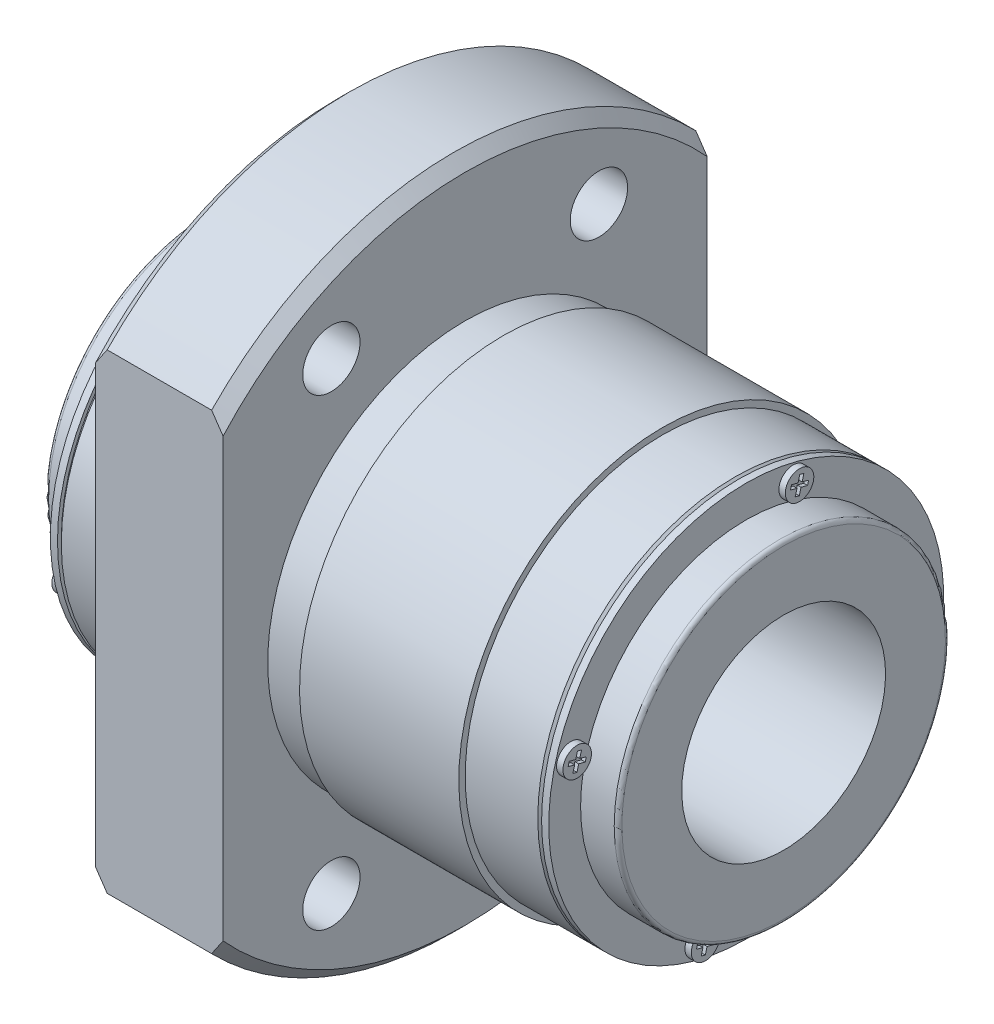
SolidWorks part; units mm, degrees
ref_plane "Front" through (0, 0, 0) normal (0, 0, 1) x (1, 0, 0)
ref_plane "Top" through (0, 0, 0) normal (0, 1, 0) x (1, 0, 0)
ref_plane "Right" through (0, 0, 0) normal (1, 0, 0) x (0, 0, -1)
sketch "Sketch1" plane through (0, 0, 0) normal (0, 0, 1) x (1, 0, 0)
  line L0 (35, 8) -> (-10, 8)
  line L1 (-10, 8) -> (-10, 13)
  line L2 (-10, 13) -> (-7.06, 13)
  line L3 (-7.06, 13) -> (-7.06, 15.5)
  line L4 (-7.06, 15.5) -> (-0.65, 15.5)
  line L5 (-0.65, 15.5) -> (-0.65, 16)
  line L6 (-0.65, 16) -> (0, 16)
  line L7 (0, 16) -> (0, 26.5)
  line L8 (0, 26.5) -> (10, 26.5)
  line L9 (10, 26.5) -> (10, 15.5)
  line L10 (10, 15.5) -> (13, 15.5)
  line L11 (13, 15.5) -> (13, 16)
  line L12 (13, 16) -> (25.5, 16)
  line L13 (25.5, 16) -> (25.5, 15.5)
  line L14 (25.5, 15.5) -> (32.06, 15.5)
  line L15 (32.06, 15.5) -> (32.06, 13)
  line L16 (32.06, 13) -> (35, 13)
  line L17 (35, 13) -> (35, 8)
  line L18 (35, 0) -> (-10, 0) construction
  dimension "D1" = 0.65
  dimension "D2" = 7.06
  dimension "D3" = 10
  dimension "D4" = 10
  dimension "D5" = 13
  dimension "D6" = 25.5
  dimension "D7" = 32.06
  dimension "D8" = 35
  dimension "D9" = 16
  dimension "D10" = 26
  dimension "D11" = 31
  dimension "D12" = 32
  dimension "D13" = 53
revolve "Revolve1" add sketch "Sketch1" angle 360 about L18
sketch "Sketch2" plane through (0, 0, 0) normal (1, 0, 0) x (0, 0, -1)
  line L0 (0, 26.5) -> (0, -26.5) construction
  line L1 (-19, 26.5) -> (19, 26.5)
  line L2 (-19, 26.5) -> (-19, -26.5)
  line L3 (-19, -26.5) -> (19, -26.5)
  line L4 (19, 26.5) -> (19, -26.5)
  circle A0 centre (0, 0) radius 26.5 construction
  dimension "D1" = 38
extrude "Cut-Extrude1" cut sketch "Sketch2" along normal through all flip side to cut
hole_wizard "Ø4.5 (4.5) Diameter Hole1" positions "Sketch5" profile "Sketch4" hole size "Ø4.5" standard "ISO" end condition through all
sketch "Sketch5" plane through (10, 0, 0) normal (1, 0, 0) x (0, 0, -1)
  line L1 (0, 26.5) -> (0, -21) construction
  circle A0 centre (0, 0) radius 21 construction
  arc A3 (19, 18.473) -> (-19, 18.473) centre (0, 0) ccw construction
  point P0 (-10.5, 18.1865)
  point P1 (-10.5, -18.1865)
  point P3 (10.5, 18.1865)
  point P5 (10.5, -18.1865)
  dimension "D1" = 42
  dimension "D2" = 21
sketch "Sketch4" plane through (10, 18.1865, 10.5) normal (0, 1, 0) x (0, 0, -1)
  line L0 (0, 0) -> (0, 20)
  line L1 (0, 20) -> (2.25, 20)
  line L2 (2.25, 20) -> (2.25, 0)
  line L5 (2.25, 0) -> (0, 0)
  line L11 (0, -6.35) -> (0, 107.95) construction
  dimension "Thru Hole Dia." = 4.5
  dimension "Thru Hole Depth" = 20
sketch "Sketch6" plane through (32.06, 0, 0) normal (1, 0, 0) x (0, 0, -1)
  line L0 (-19, 0) -> (19, 0) construction
  line L1 (0, 26.5) -> (0, -26.5) construction
  line L2 (-18.1829, 4.8721) -> (18.5076, -4.9591) construction
  line L3 (-4.9176, -18.3528) -> (4.686, 17.4885) construction
  line L4 (-19, -18.473) -> (-19, 18.473) construction
  line L5 (19, 18.473) -> (19, -18.473) construction
  circle A0 centre (0, 0) radius 14.25 construction
  circle A3 centre (3.6882, 13.7644) radius 1.12
  circle A4 centre (-13.7644, 3.6882) radius 1.12
  circle A5 centre (-3.6882, -13.7644) radius 1.12
  circle A6 centre (13.7644, -3.6882) radius 1.12
  arc A7 (19, 18.473) -> (-19, 18.473) centre (0, 0) ccw construction
  arc A8 (-19, -18.473) -> (19, -18.473) centre (0, 0) ccw construction
  dimension "D1" = 28.5
  dimension "D2" = 2.24
  dimension "D3" = 15
  dimension "D4" = 75
extrude "Boss-Extrude1" add sketch "Sketch6" along normal blind 0.5
sketch "Sketch7" plane through (32.56, 0, 0) normal (1, 0, 0) x (0, 0, -1)
  line L0 (-4.9176, -18.3528) -> (4.686, 17.4885) construction
  line L1 (4.0274, 14.3931) -> (3.7087, 14.4785)
  line L2 (4.0274, 14.3931) -> (3.8903, 13.8811)
  line L3 (3.6677, 13.0504) -> (3.3489, 13.1358)
  line L4 (3.7087, 14.4785) -> (3.5715, 13.9665)
  line L5 (4.0274, 14.3931) -> (3.3489, 13.1358) construction
  line L6 (3.6677, 13.0504) -> (3.7087, 14.4785) construction
  line L7 (3.4861, 13.6478) -> (3.3489, 13.1358)
  line L8 (3.0596, 14.1037) -> (3.5715, 13.9665)
  line L9 (3.0596, 14.1037) -> (2.9741, 13.7849)
  line L10 (2.9741, 13.7849) -> (3.4861, 13.6478)
  line L11 (4.4022, 13.7439) -> (4.3168, 13.4252)
  line L12 (3.0596, 14.1037) -> (4.3168, 13.4252) construction
  line L13 (2.9741, 13.7849) -> (4.4022, 13.7439) construction
  line L14 (3.8903, 13.8811) -> (4.4022, 13.7439)
  line L15 (3.8048, 13.5624) -> (3.6677, 13.0504)
  line L16 (3.8048, 13.5624) -> (4.3168, 13.4252)
  line L48 (0, 26.5) -> (0, -26.5) construction
  arc A0 (19, 18.473) -> (-19, 18.473) centre (0, 0) ccw construction
  arc A1 (-19, -18.473) -> (19, -18.473) centre (0, 0) ccw construction
  point P0 (3.6882, 13.7644)
  point P7 (3.6882, 13.7644)
  dimension "D1" = 0.33
  dimension "D2" = 1.39
  dimension "D3" = 1.39
extrude "Cut-Extrude2" cut sketch "Sketch7" against normal blind 0.3
pattern_circular "CirPattern1" count 4 over 360 about axis through (0, 0, 0) along (1, 0, 0) of "Cut-Extrude2"
sketch "Sketch8" plane through (-7.06, 0, 0) normal (-1, 0, 0) x (0, 0, 1)
  line L0 (0, 26.5) -> (0, -26.5) construction
  line L1 (19, 0) -> (-19, 0) construction
  line L2 (0, 26.5) -> (0, -26.5) construction
  line L3 (19, 0) -> (-19, 0) construction
  line L4 (-17.1718, 4.6012) -> (16.887, -4.5249) construction
  line L5 (-4.825, -18.007) -> (4.3771, 16.3354) construction
  circle A4 centre (3.6882, 13.7644) radius 1.12
  circle A5 centre (-13.7644, 3.6882) radius 1.12
  circle A6 centre (-3.6882, -13.7644) radius 1.12
  circle A7 centre (13.7644, -3.6882) radius 1.12
  circle A8 centre (0, 0) radius 14.25 construction
  circle A9 centre (0, 0) radius 14.25 construction
  dimension "D3" = 2.24
  dimension "D1" = 15
  dimension "D2" = 75
extrude "Boss-Extrude2" add sketch "Sketch8" along normal blind 0.5
sketch "Sketch9" plane through (-7.56, 0, 0) normal (-1, 0, 0) x (0, 0, 1)
  line L0 (3.5715, 13.9665) -> (3.7087, 14.4785)
  line L1 (3.8903, 13.8811) -> (4.0274, 14.3931)
  line L2 (3.4861, 13.6478) -> (2.9741, 13.7849)
  line L3 (3.5715, 13.9665) -> (3.0596, 14.1037)
  line L34 (-4.825, -18.007) -> (4.3771, 16.3354) construction
  line L35 (3.3489, 13.1358) -> (3.6677, 13.0504)
  line L36 (3.3489, 13.1358) -> (3.4861, 13.6478)
  line L37 (3.7087, 14.4785) -> (4.0274, 14.3931)
  line L38 (3.6677, 13.0504) -> (3.8048, 13.5624)
  line L39 (3.3489, 13.1358) -> (4.0274, 14.3931) construction
  line L40 (3.7087, 14.4785) -> (3.6677, 13.0504) construction
  line L42 (4.3168, 13.4252) -> (3.8048, 13.5624)
  line L43 (4.3168, 13.4252) -> (4.4022, 13.7439)
  line L44 (4.4022, 13.7439) -> (3.8903, 13.8811)
  line L45 (2.9741, 13.7849) -> (3.0596, 14.1037)
  line L46 (4.3168, 13.4252) -> (3.0596, 14.1037) construction
  line L47 (4.4022, 13.7439) -> (2.9741, 13.7849) construction
  point P0 (3.6882, 13.7644)
  point P7 (3.6882, 13.7644)
  dimension "D1" = 0.33
  dimension "D2" = 1.39
  dimension "D3" = 1.39
extrude "Cut-Extrude3" cut sketch "Sketch9" against normal blind 0.3
pattern_circular "CirPattern2" count 4 over 360 about axis through (0, 0, 0) along (1, 0, 0) of "Cut-Extrude3"
ref_plane "Plane1" through (0, -26.5, 0) normal (0, -1, 0) x (1, 0, 0)
hole_wizard "M6 Tapped Hole1" positions "Sketch11" profile "Sketch10" tap size "M6" standard "ISO"
sketch "Sketch11" plane through (0, -26.5, 0) normal (0, -1, 0) x (1, 0, 0)
  line L0 (-3.1372, 0) -> (12.0083, 0) construction
  point P1 (5, 0)
  dimension "D1" = 5
sketch "Sketch10" plane through (5, -26.5, 0) normal (1, 0, 0) x (0, 0, -1)
  line L0 (0, 0) -> (0, 12.5022)
  line L1 (0, 12.5022) -> (2.5, 11)
  line L2 (2.5, 11) -> (2.5, 0)
  line L5 (2.5, 0) -> (0, 0)
  line L10 (0, 12.5022) -> (-2.5, 11) construction
  line L11 (0, -6.35) -> (0, 107.95) construction
  dimension "Tap Drill Dia." = 5
  dimension "Tap Drill Depth" = 11
  dimension "Drill Angle" = 118
cosmetic thread "Hole Thread1" parameters "D1"=8, "D2"=6
sketch "Sketch12" plane through (0, 0, 0) normal (0, 1, 0) x (1, 0, 0)
  line L0 (31.2, -15.5) -> (31.5, -15.2)
  line L1 (25.5, -15.5) -> (32.06, -15.5) construction
  line L2 (31.5, -15.2) -> (31.5, -15.5)
  line L3 (25.5, -15.5) -> (32.06, -15.5) construction
  line L4 (31.5, -15.5) -> (31.2, -15.5)
  line L5 (-12.4047, 0) -> (38.4306, 0) construction
  line L6 (-6.5, -15.5) -> (-6.5, -15.2)
  line L7 (-7.06, -15.5) -> (-0.65, -15.5) construction
  line L8 (-6.5, -15.2) -> (-6.2, -15.5)
  line L9 (-7.06, -15.5) -> (-0.65, -15.5) construction
  line L10 (-6.2, -15.5) -> (-6.5, -15.5)
  dimension "D1" = 31.5
  dimension "D2" = 30.4
  dimension "D3" = 45
  dimension "D4" = 6.5
revolve "Cut-Revolve1" cut sketch "Sketch12" angle 360 mid plane about L5
chamfer "Chamfer1" distance 0.9 angle 45 4 edges at (0, 26.5, 0) (0, -26.5, 0) (10, -26.5, 0) (10, 26.5, 0)
fillet "Fillet1" radius 0.3 2 edges at (35, 13, 0) (-10, 13, 0)
